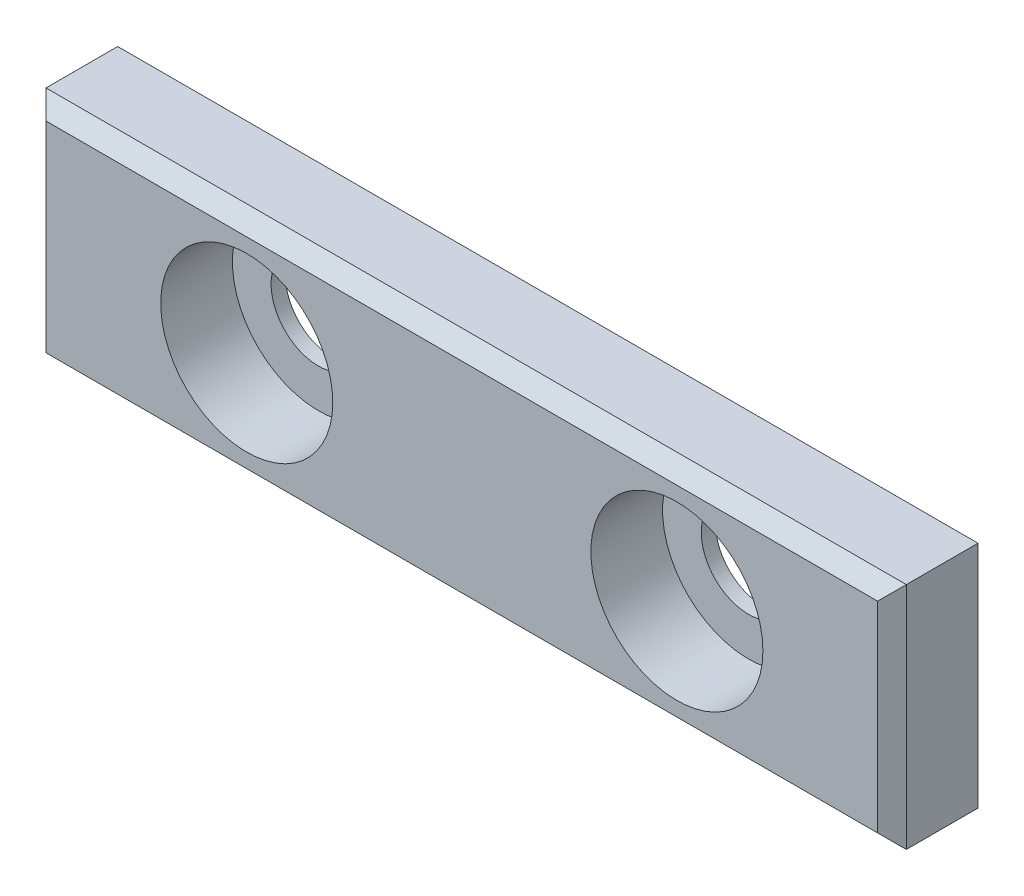
SolidWorks part; units mm, degrees
material "镍"
ref_plane "Front view" through (0, 0, 0) normal (0, 0, 1) x (1, 0, 0)
ref_plane "Top view" through (0, 0, 0) normal (0, 1, 0) x (1, 0, 0)
ref_plane "Right view" through (0, 0, 0) normal (1, 0, 0) x (0, 0, -1)
sketch "Sketch1" plane through (0, 0, 0) normal (0, 0, 1) x (1, 0, 0)
  line L1 (-12.6282, 5.7395) -> (47.3718, 5.7395)
  line L2 (-12.6282, 5.7395) -> (-12.6282, -10.2605)
  line L3 (-12.6282, -10.2605) -> (47.3718, -10.2605)
  line L4 (47.3718, 5.7395) -> (47.3718, -10.2605)
  dimension "D1" = 60
  dimension "D2" = 16
extrude "Base-Extrude" add sketch "Sketch1" along normal blind 6
sketch "Sketch2" plane through (0, 0, 6) normal (0, 0, 1) x (1, 0, 0)
  line L0 (2.3718, 4.5437) -> (2.3718, -11.9817) construction
  line L1 (-13.6358, -2.2605) -> (-2.5247, -2.2605) construction
  line L2 (-12.6282, 5.7395) -> (-12.6282, -10.2605) construction
  line L3 (47.3718, 5.7395) -> (-12.6282, 5.7395) construction
  circle A0 centre (2.3718, -2.2605) radius 3.3
  dimension "D3" = 6.6
  dimension "D1" = 15
  dimension "D2" = 8
extrude "Cut-Extrude1" cut sketch "Sketch2" against normal through all
sketch "Sketch3" plane through (0, 0, 6) normal (0, 0, 1) x (1, 0, 0)
  line L0 (2.3718, 4.2048) -> (2.3718, 3.6177) construction
  line L1 (2.3718, 3.9112) -> (2.3718, -11.0608) construction
  line L2 (-13.2839, -2.2605) -> (1.1988, -2.2605) construction
  line L3 (-12.6282, 5.7395) -> (-12.6282, -10.2605) construction
  line L4 (-12.6282, -10.2605) -> (47.3718, -10.2605) construction
  circle A0 centre (2.3718, -2.2605) radius 6
  dimension "D3" = 12
  dimension "D1" = 15
  dimension "D2" = 8
extrude "Cut-Extrude2" cut sketch "Sketch3" against normal blind 5
pattern_linear "LPattern1" count 2 spacing 30 along (1, 0, 0) of "Cut-Extrude1", "Cut-Extrude2"
chamfer "Chamfer1" distance 1 angle 45 4 edges at (47.3718, -2.2605, 6) (17.3718, 5.7395, 6) (-12.6282, -2.2605, 6) (17.3718, -10.2605, 6)
